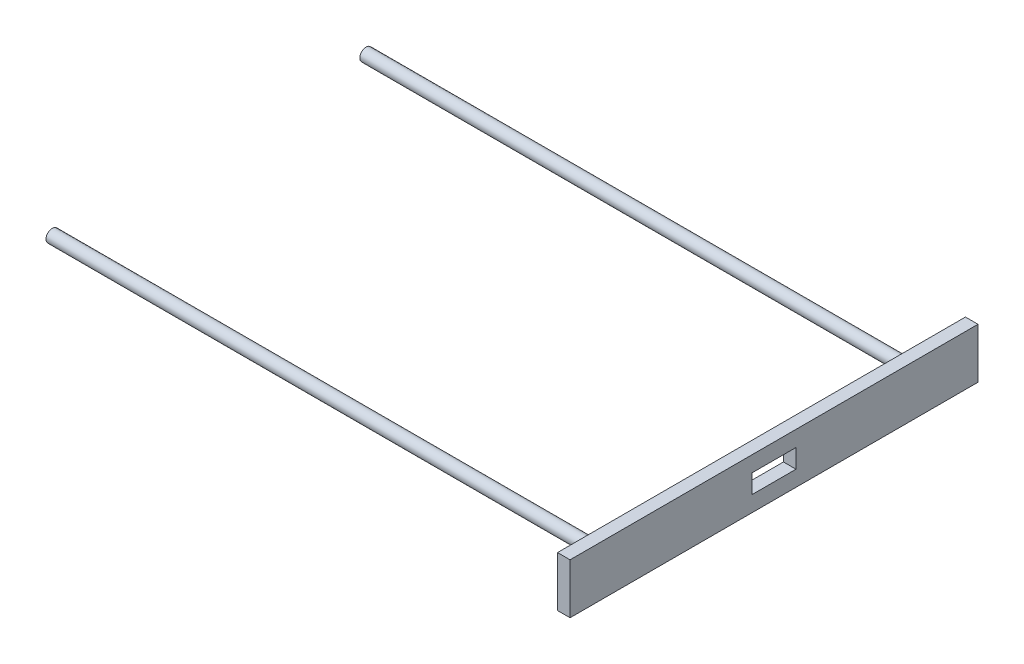
from build123d import *

# Parameters (mm, degrees)
SKETCH1_W           = 660
SKETCH1_H           = 90
SKETCH1_R           = 10
SKETCH1_W_2         = 70
SKETCH1_H_2         = 30
BOSS_EXTRUDE1_DEPTH = 20
BOSS_EXTRUDE2_START = -900
SKETCH2_R           = 10
BOSS_EXTRUDE2_DEPTH = 900
SKETCH3_W           = 903.641141734
SKETCH3_H           = 235.635140662
SKETCH3_W_2         = 650
SKETCH3_H_2         = 80
CUT_EXTRUDE1_DEPTH  = 960.648373103


with BuildPart() as part:
    # Sketch1 → Boss-Extrude1 (new body)
    with BuildSketch(Plane(origin=(0, 0, 0), x_dir=(0, 0, -1), z_dir=(1, 0, 0))):
        Rectangle(SKETCH1_W, SKETCH1_H)
        with Locations((-250, 0)):
            Circle(SKETCH1_R, mode=Mode.SUBTRACT)
        with Locations((250, 0)):
            Circle(SKETCH1_R, mode=Mode.SUBTRACT)
        Rectangle(SKETCH1_W_2, SKETCH1_H_2, mode=Mode.SUBTRACT)
    extrude(amount=BOSS_EXTRUDE1_DEPTH)

    # Sketch2 → Boss-Extrude2 (add)
    with BuildSketch(Plane(origin=(20, 0, 0), x_dir=(0, 0, -1), z_dir=(1, 0, 0)).offset(BOSS_EXTRUDE2_START)):
        with Locations((-250, 0)):
            Circle(SKETCH2_R)
        with Locations((250, 0)):
            Circle(SKETCH2_R)
    extrude(amount=BOSS_EXTRUDE2_DEPTH)

    # Sketch3 → Cut-Extrude1 (cut, through all)
    with BuildSketch(Plane(origin=(20, 0, 0), x_dir=(0, 0, -1), z_dir=(1, 0, 0))):
        Rectangle(SKETCH3_W, SKETCH3_H)
        Rectangle(SKETCH3_W_2, SKETCH3_H_2, mode=Mode.SUBTRACT)
    extrude(amount=-CUT_EXTRUDE1_DEPTH, mode=Mode.SUBTRACT)


solid = part.part
